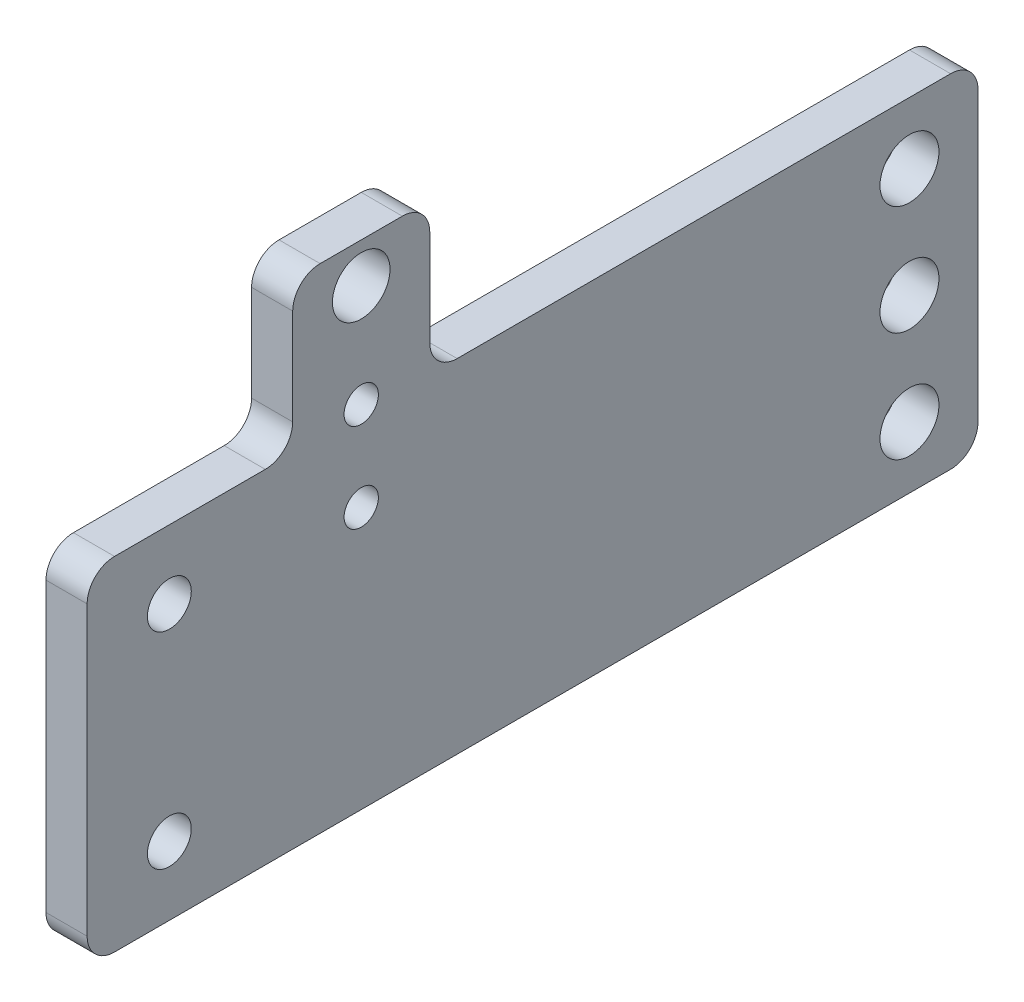
from build123d import *

# Parameters (mm, degrees)
SKETCH_1_W                  = 65
SKETCH_1_H                  = 25
SKETCH_1_R                  = 1.6
EXTRUDE_1_DEPTH             = 3
FILLET_1_R                  = 2
HOLE_WIZARD_4_3_4_3_1_D     = 4.3
HOLE_WIZARD_4_3_4_3_1_DEPTH = 11.5
HOLE_WIZARD_4_3_4_3_1_TIP   = 1.291850331
SKETCH_4_W                  = 10
SKETCH_4_H                  = 22
EXTRUDE_2_DEPTH             = 3
SKETCH_5_R                  = 2.1
CUT_EXTRUDE_1_DEPTH         = 10
FILLET_2_R                  = 2
HOLE_WIZARD_M3_1_D          = 2.5
HOLE_WIZARD_M3_1_DEPTH      = 8.5
HOLE_WIZARD_M3_1_TIP        = 0.751075774


with BuildPart() as part:
    # 草图1 → 凸台-拉伸1 (new body)
    with BuildSketch(Plane(origin=(0, 0, 0), x_dir=(0, 0, -1), z_dir=(1, 0, 0))):
        Rectangle(SKETCH_1_W, SKETCH_1_H)
        with Locations((-26.5, 7.5)):
            Circle(SKETCH_1_R, mode=Mode.SUBTRACT)
        with Locations(Location((-26.5, -7.5, 0), (0, 0, 180))):
            Circle(SKETCH_1_R, mode=Mode.SUBTRACT)
    extrude(amount=EXTRUDE_1_DEPTH)

    # 圆角1
    fillet_1_edges = [part.edges().sort_by_distance(p)[0] for p in [
        (1.5, -12.5, -32.5),
        (1.5, -12.5, 32.5),
        (1.5, 12.5, 32.5),
        (1.5, 12.5, -32.5),
    ]]
    fillet(fillet_1_edges, radius=FILLET_1_R)

    # Ø4.3 (4.3) 直径孔1
    with Locations(Plane.ZY):
        with Locations((-27.5, 8), (-27.5, -8), (-27.5, 0)):
            Hole(HOLE_WIZARD_4_3_4_3_1_D / 2, depth=HOLE_WIZARD_4_3_4_3_1_DEPTH)
            with Locations((0, 0, -(HOLE_WIZARD_4_3_4_3_1_DEPTH + HOLE_WIZARD_4_3_4_3_1_TIP / 2))):  # 118° drill point
                Cone(0, HOLE_WIZARD_4_3_4_3_1_D / 2, HOLE_WIZARD_4_3_4_3_1_TIP, mode=Mode.SUBTRACT)

    # 草图4 → 凸台-拉伸2 (add)
    with BuildSketch(Plane(origin=(3, 0, 0), x_dir=(0, 0, -1), z_dir=(1, 0, 0))):
        with Locations((-12.5, 12.5)):
            Rectangle(SKETCH_4_W, SKETCH_4_H)
    extrude(amount=-EXTRUDE_2_DEPTH)

    # 草图5 → 切除-拉伸1 (cut)
    with BuildSketch(Plane.ZY):
        with Locations((12.5, 20.6)):
            Circle(SKETCH_5_R)
    extrude(amount=-CUT_EXTRUDE_1_DEPTH, mode=Mode.SUBTRACT)

    # 圆角2
    fillet_2_edges = [part.edges().sort_by_distance(p)[0] for p in [
        (1.5, 12.5, 17.5),
        (1.5, 12.5, 7.5),
        (1.5, 23.5, 7.5),
        (1.5, 23.5, 17.5),
    ]]
    fillet(fillet_2_edges, radius=FILLET_2_R)

    # M3 螺纹孔1
    with Locations(Plane.ZY):
        with Locations((12.5, 6.6), (12.5, 13.1)):
            Hole(HOLE_WIZARD_M3_1_D / 2, depth=HOLE_WIZARD_M3_1_DEPTH)
            with Locations((0, 0, -(HOLE_WIZARD_M3_1_DEPTH + HOLE_WIZARD_M3_1_TIP / 2))):  # 118° drill point
                Cone(0, HOLE_WIZARD_M3_1_D / 2, HOLE_WIZARD_M3_1_TIP, mode=Mode.SUBTRACT)


solid = part.part
